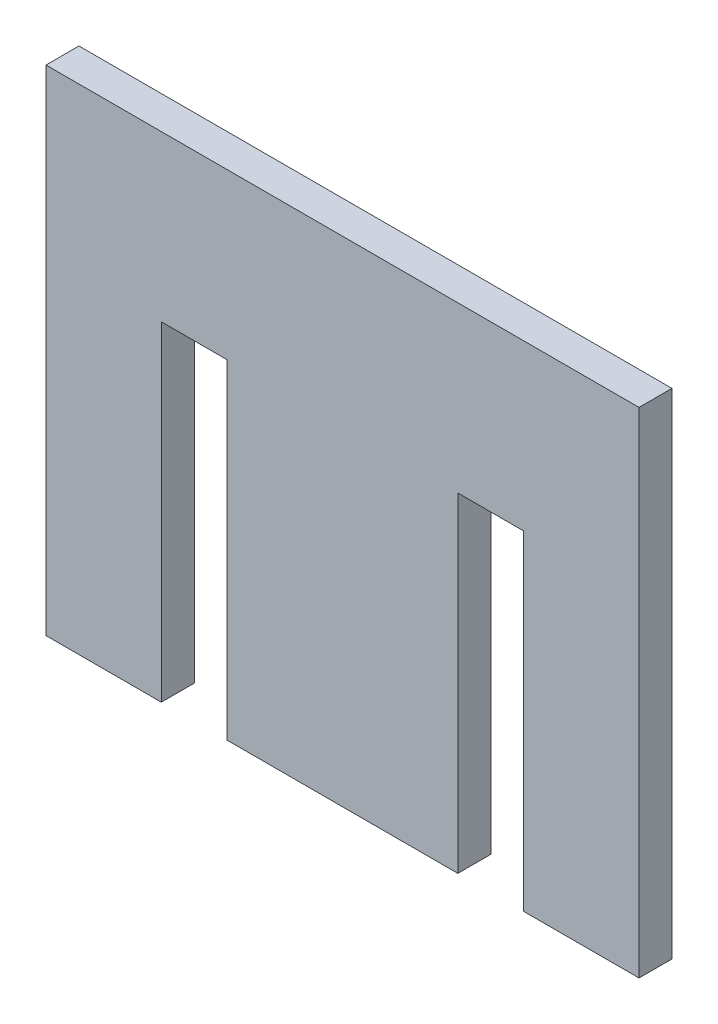
from build123d import *

# Parameters (mm, degrees)
SKETCH_1_W          = 180
SKETCH_1_H          = 150
EXTRUDE_1_DEPTH     = 10
CUT_EXTRUDE_1_REACH = 119.58
SKETCH_2_W          = 20
SKETCH_2_H          = 100


with BuildPart() as part:
    # 草图1 → 凸台-拉伸1 (new body)
    with BuildSketch(Plane.XY):
        Rectangle(SKETCH_1_W, SKETCH_1_H)
    extrude(amount=EXTRUDE_1_DEPTH)

    # 草图2 → 切除-拉伸1 (cut, up to next)
    with BuildSketch(Plane.XY.offset(10), mode=Mode.PRIVATE) as cut_extrude_1_sk1:
        with Locations((-45, -25)):
            Rectangle(SKETCH_2_W, SKETCH_2_H)
    cut_extrude_1_tool1 = extrude(cut_extrude_1_sk1.sketch, amount=-CUT_EXTRUDE_1_REACH, mode=Mode.PRIVATE) & part.part
    cut_extrude_1 = cut_extrude_1_tool1.solids().sort_by_distance((-45, -25, 10))[0]
    add(cut_extrude_1, mode=Mode.SUBTRACT)

    # 镜向1: 切除-拉伸1 across plane
    add(cut_extrude_1.mirror(Plane(origin=(0, 0, 0), x_dir=(0, 0, 1), z_dir=(1, 0, 0))), mode=Mode.SUBTRACT)


solid = part.part
